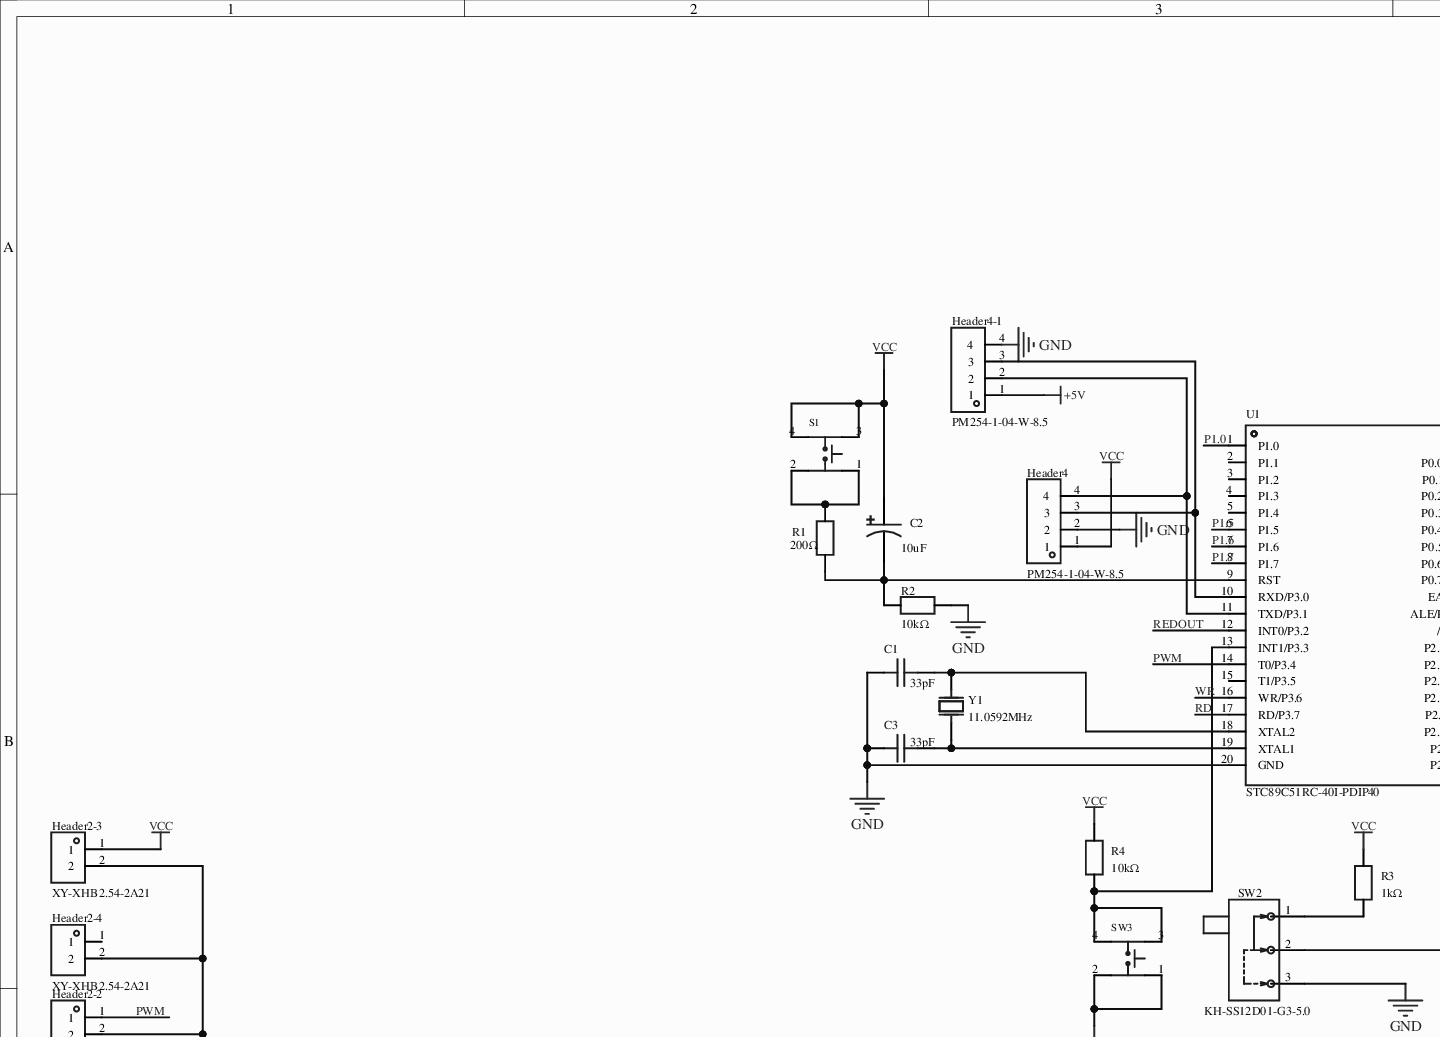
[diagram p0: MISC52142-3.schdoc, top left]
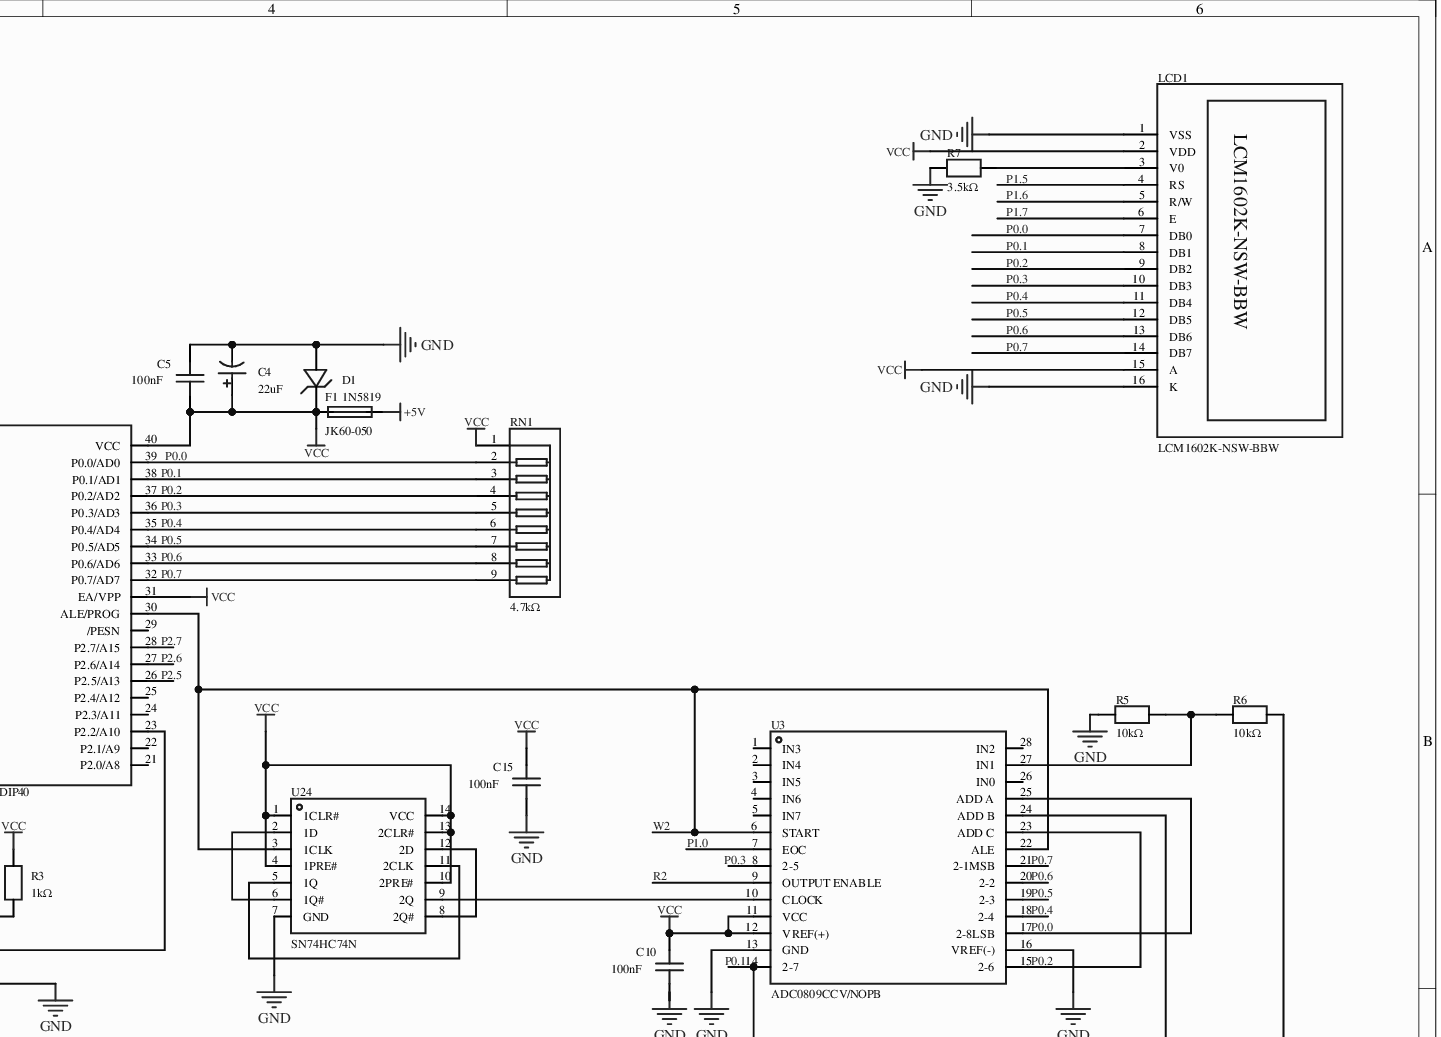
[diagram p1: MISC52142-3.schdoc, top right]
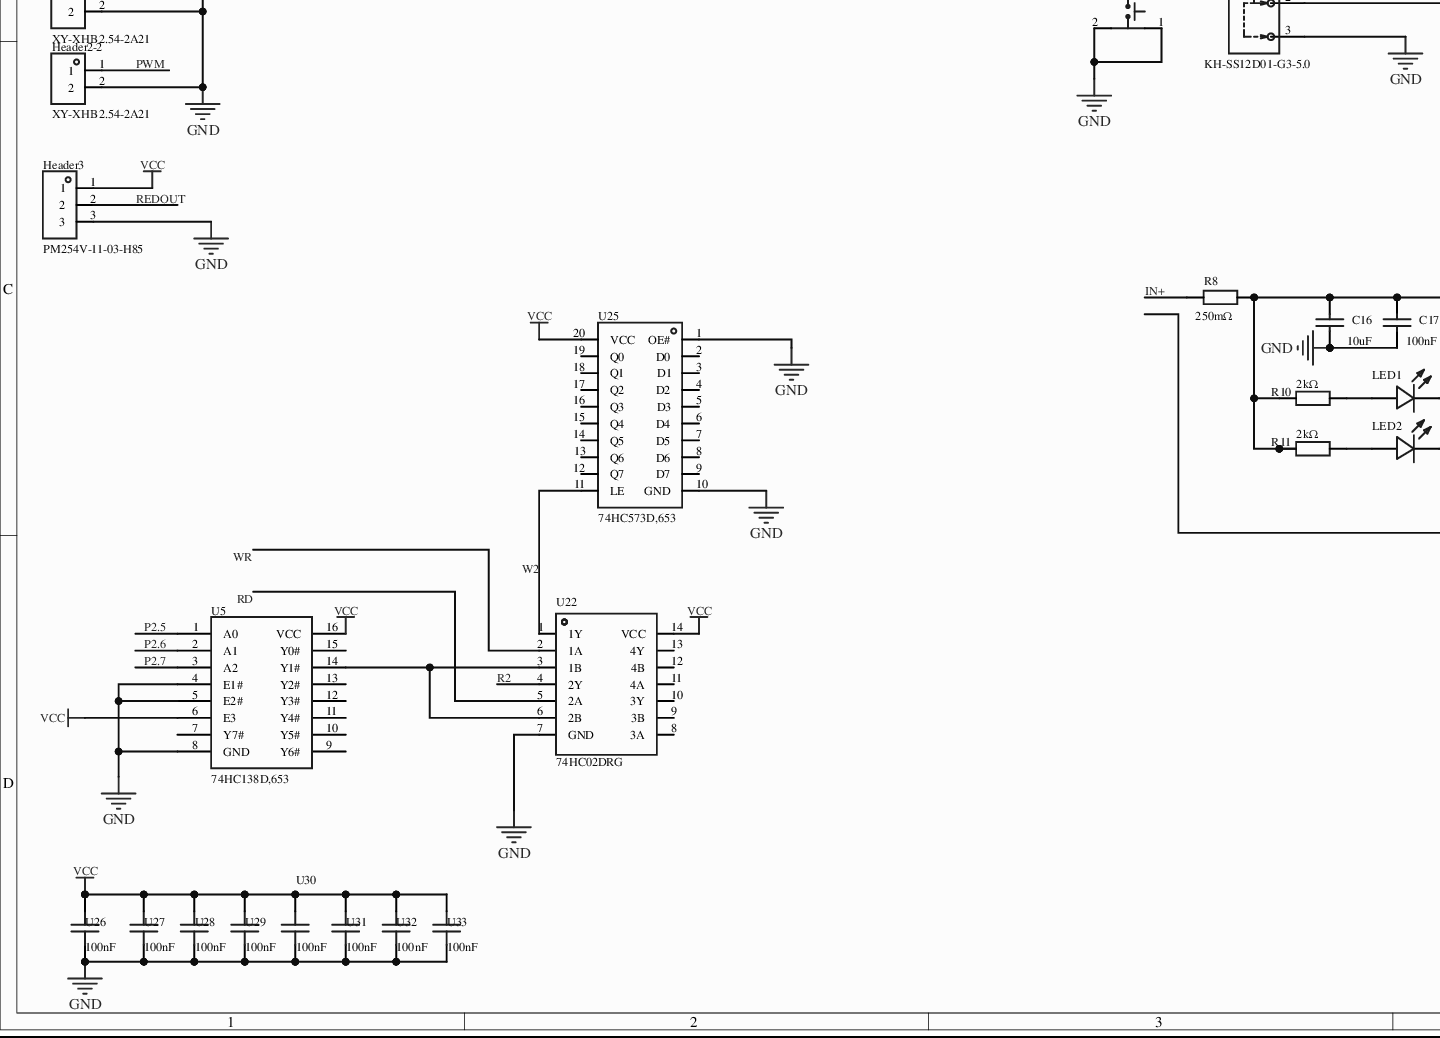
[diagram p2: MISC52142-3.schdoc, bottom left]
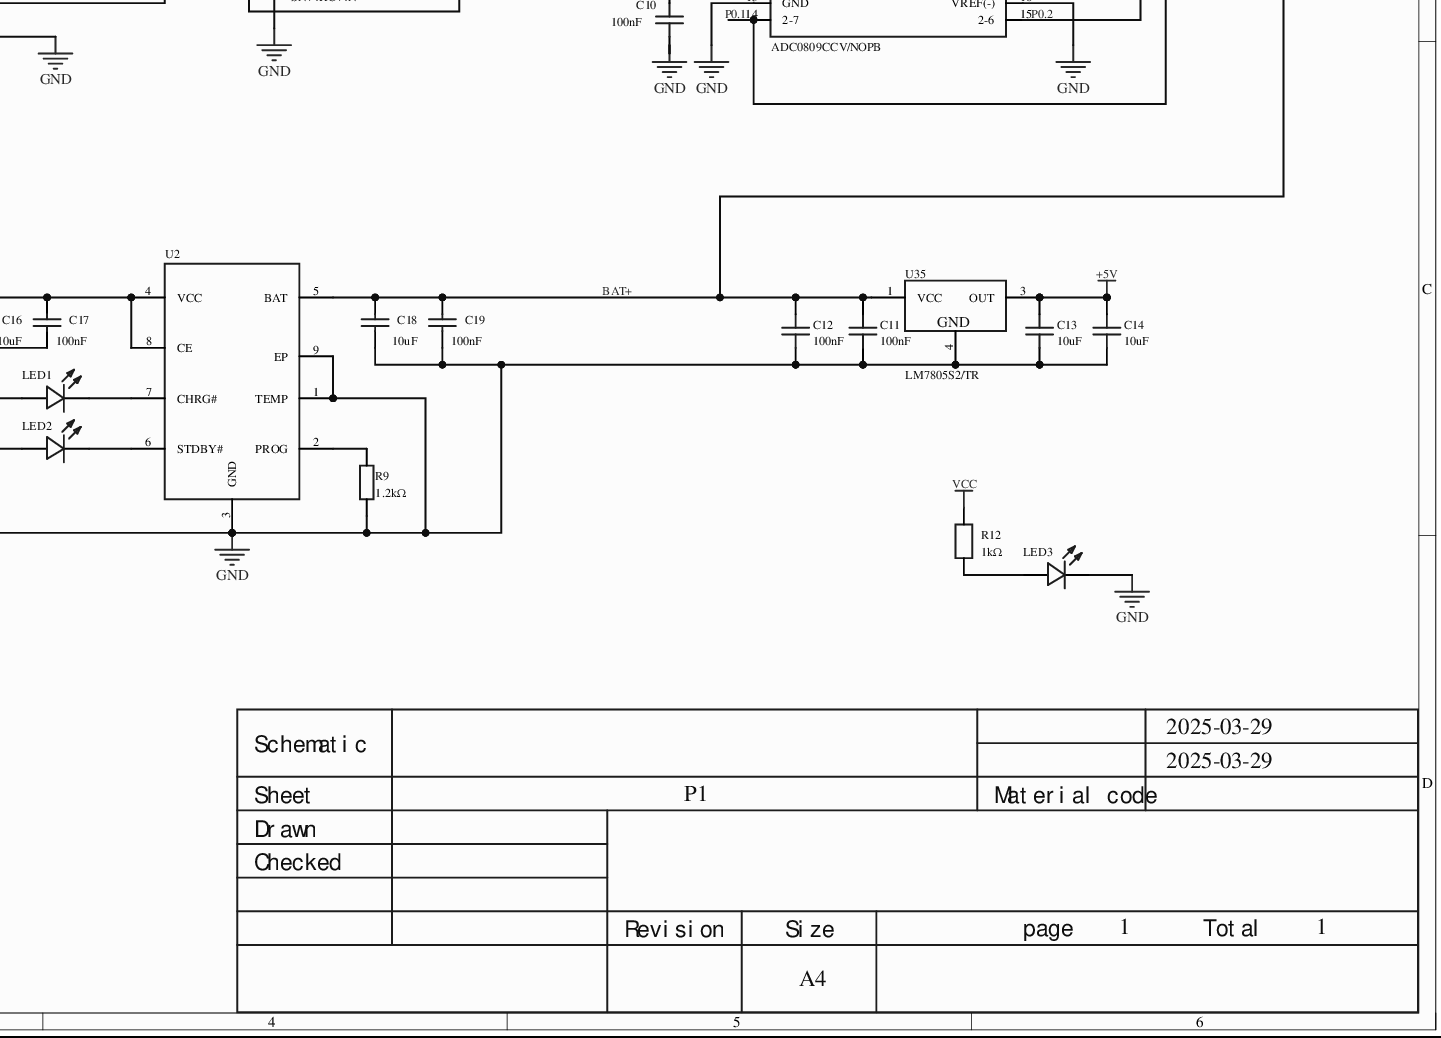
[diagram p3: MISC52142-3.schdoc, bottom right]
# Altium project MISC52142-2.PrjPcb
1 sheet, 60 parts. Net scope: global (net labels, ports and power ports of the same name join across sheets).
Board file: MISC52142.pcbdoc

## Sheet MISC52142-3.schdoc
size 420 x 298 mm; Version: V1.0; @Project Name: MISC52142; @Page Count: 1; @Update Date: 2025-03-29; @Create Date: 2025-03-29; @Schematic Name: MISC52142; @Page No: 1

### Parts
C1  33pF  [RAD-0.2]
C2  10uF  [RB1-2]
C3  33pF  [RAD-0.2]
C4  22uF  [RB1-2]
C5  100nF  [RAD-0.2]
C10  100nF  [RAD-0.2]
C11  100nF  [RAD-0.2]
C12  100nF  [RAD-0.2]
C13  10uF  [RAD-0.2]
C14  10uF  [RAD-0.2]
C15  100nF  [RAD-0.2]
C16  10uF  [RAD-0.2]
C17  100nF  [RAD-0.2]
C18  10uF  [RAD-0.2]
C19  100nF  [RAD-0.2]
D1  1N5819  [DIODE-3]
F1  JK60-050  [FUSE-2]
Header2-2  XY-XHB2.54-2A21  [CON2-5]
Header2-3  XY-XHB2.54-2A21  [CON2-5]
Header2-4  XY-XHB2.54-2A21  [CON2-5]
Header3  PM254V-11-03-H85  [CON3]
Header4  PM254-1-04-W-8.5  [CON4]
Header4-1  PM254-1-04-W-8.5  [CON4]
LCD1  LCM1602K-NSW-BBW  [LCD1602]
LED1  204-10SYGD/S530-E3  [LED1]  (value not drawn)
LED2  333-2SYGD/S530-E2-L  [LED1]  (value not drawn)
LED3  204-10SYGD/S530-E3  [LED1]  (value not drawn)
R1  200Ω  [AXIAL-0.3]
R2  10kΩ  [AXIAL-0.3]
R3  1kΩ  [AXIAL-0.3]
R4  10kΩ  [AXIAL-0.3]
R5  10kΩ  [AXIAL-0.3]
R6  10kΩ  [AXIAL-0.3]
R7  3.5kΩ  [AXIAL-0.3]
R8  250mΩ  [AXIAL-0.3]
R9  1.2kΩ  [AXIAL-0.3]
R10  2kΩ  [AXIAL-0.3]
R11  2kΩ  [AXIAL-0.3]
R12  1kΩ  [AXIAL-0.3]
RN1  4.7kΩ  [RP]
S1  (no value)  [RST]
SW2  KH-SS12D01-G3-5.0  [RT]
SW3  (no value)  [RST]
U1  STC89C51RC-40I-PDIP40  [DIP-40]
U2  TP4056-42-ESOP8  [ESOP-8_L4.9-W3.9-P1.27-LS6.0-BL-EP]  (value not drawn)
U3  ADC0809CCV/NOPB  [DIP-28]
U5  74HC138D,653  [DIP-16]
U22  74HC02DRG  [DIP-14]
U24  SN74HC74N  [DIP-14]
U25  74HC573D,653  [DIP-20]
U26  100nF  [RAD-0.2]
U27  100nF  [RAD-0.2]
U28  100nF  [RAD-0.2]
U29  100nF  [RAD-0.2]
U30  100nF  [RAD-0.2]
U31  100nF  [RAD-0.2]
U32  100nF  [RAD-0.2]
U33  100nF  [RAD-0.2]
U35  LM7805S2/TR  [TO-263-2_L10.0-W9.1-P5.08-LS15.2-BL]
Y1  11.0592MHz  [XTAL-2]

### Nets
+5V: C13.2 C14.2 F1.2 Header4-1.1 U35.3(OUT)
GND: C1.2 C3.2 C4.2 C5.2 C10.1 C11.1 C12.1 C13.1 C14.1 C15.1 C16.1 C17.1 C18.1 C19.1 D1.2(A) Header2-2.2 Header2-3.2 Header2-4.2 Header3.3 Header4.2 Header4-1.4 LCD1.1(VSS) LCD1.16(K) LED3.2(-) R2.2 R5.1 R7.1 R9.1 SW2.3 SW3.1 SW3.2 U1.20(GND) U2.1(TEMP) U2.3(GND) U2.9(EP) U3.13(GND) U3.16(VREF(-)) U5.4(E1#) U5.5(E2#) U5.8(GND) U22.7(GND) U24.7(GND) U25.1(OE#) U25.10(GND) U26.1 U27.1 U28.1 U29.1 U30.1 U31.1 U32.1 U33.1 U35.4(GND)
VCC: C2.1 C4.1 C5.1 C10.2 C15.2 D1.1(C) F1.1 Header2-3.1 Header3.1 Header4.1 LCD1.2(VDD) LCD1.15(A) R3.2 R4.2 R12.2 RN1.1 S1.3 S1.4 U1.31(EA/VPP) U1.40(VCC) U3.11(VCC) U3.12(VREF(+)) U5.6(E3) U5.16(VCC) U22.14(VCC) U24.1(1CLR#) U24.4(1PRE#) U24.10(2PRE#) U24.13(2CLR#) U24.14(VCC) U25.20(VCC) U26.2 U27.2 U28.2 U29.2 U30.2 U31.2 U32.2 U33.2
BAT+: C11.2 C12.2 C18.2 C19.2 R6.2 U2.5(BAT) U35.1(VCC)
IN+: R8.1
P0.0: LCD1.7(DB0) RN1.2 U1.39(P0.0/AD0) U3.17(2-8LSB) U3.25(ADD_A)
P0.1: LCD1.8(DB1) RN1.3 U1.38(P0.1/AD1) U3.14(2-7) U3.24(ADD_B)
P0.2: LCD1.9(DB2) RN1.4 U1.37(P0.2/AD2) U3.15(2-6) U3.23(ADD_C)
P0.3: LCD1.10(DB3) RN1.5 U1.36(P0.3/AD3) U3.8(2-5)
P0.4: LCD1.11(DB4) RN1.6 U1.35(P0.4/AD4) U3.18(2-4)
P0.5: LCD1.12(DB5) RN1.7 U1.34(P0.5/AD5) U3.19(2-3)
P0.6: LCD1.13(DB6) RN1.8 U1.33(P0.6/AD6) U3.20(2-2)
P0.7: LCD1.14(DB7) RN1.9 U1.32(P0.7/AD7) U3.21(2-1MSB)
P1.0: U1.1(P1.0) U3.7(EOC)
P1.5: LCD1.4(RS) U1.6(P1.5)
P1.6: LCD1.5(R/W) U1.7(P1.6)
P1.7: LCD1.6(E) U1.8(P1.7)
P2.5: U1.26(P2.5/A13) U5.1(A0)
P2.6: U1.27(P2.6/A14) U5.2(A1)
P2.7: U1.28(P2.7/A15) U5.3(A2)
PWM: Header2-2.1 U1.14(T0/P3.4)
R2: U3.9(OUTPUT_ENABLE) U22.4(2Y)
RD: U1.17(RD/P3.7) U22.5(2A)
REDOUT: Header3.2 U1.12(INT0/P3.2)
W2: U1.30(ALE/PROG) U3.6(START) U3.22(ALE) U22.1(1Y) U24.3(1CLK) U25.11(LE)
WR: U1.16(WR/P3.6) U22.2(1A)
NetC1_1: C1.1 U1.18(XTAL2) Y1.1(OSC1)
NetC2_2: C2.2 R1.2 R2.1 U1.9(RST)
NetC3_1: C3.1 U1.19(XTAL1) Y1.2(OSC2)
NetC16_2: C16.2 C17.2 R8.2 R10.1 R11.1 U2.4(VCC) U2.8(CE)
NetHeader4_3: Header4.3 Header4-1.3 U1.10(RXD/P3.0)
NetHeader4_4: Header4.4 Header4-1.2 U1.11(TXD/P3.1)
NetLCD1_3: LCD1.3(V0) R7.2
NetLED1_1: LED1.1(+) R10.2
NetLED1_2: LED1.2(-) U2.7(CHRG#)
NetLED2_1: LED2.1(K) U2.6(STDBY#)
NetLED2_2: LED2.2(A) R11.2
NetLED3_1: LED3.1(+) R12.1
NetR1_1: R1.1 S1.1 S1.2
NetR3_1: R3.1 SW2.1
NetR4_1: R4.1 SW3.3 SW3.4 U1.13(INT1/P3.3)
NetR5_2: R5.2 R6.1 U3.27(IN1)
NetR9_2: R9.2 U2.2(PROG)
NetSW2_2: SW2.2 U1.23(P2.2/A10)
NetU3_10: U3.10(CLOCK) U24.9(2Q)
NetU5_14: U5.14(Y1#) U22.3(1B) U22.6(2B)
NetU24_2: U24.2(1D) U24.6(1Q#)
NetU24_5: U24.5(1Q) U24.11(2CLK)
NetU24_8: U24.8(2Q#) U24.12(2D)

Not connected (* = marked no-connect by the designer): Header2-4 1; U1 2(P1.1) 3(P1.2) 4(P1.3) 5(P1.4) 15(T1/P3.5) 21(P2.0/A8) 22(P2.1/A9) 24(P2.3/A11) 25(P2.4/A12) 29(/PESN); U3 1(IN3) 2(IN4) 3(IN5) 4(IN6) 5(IN7) 26(IN0) 28(IN2); U5 7(Y7#) 9(Y6#) 10(Y5#) 11(Y4#) 12(Y3#) 13(Y2#) 15(Y0#); U22 8(3A) 9(3B) 10(3Y) 11(4A) 12(4B) 13(4Y); U25 2(D0) 3(D1) 4(D2) 5(D3) 6(D4) 7(D5) 8(D6) 9(D7) 12(Q7) 13(Q6) 14(Q5) 15(Q4) 16(Q3) 17(Q2) 18(Q1) 19(Q0)

### Notes on the sheet
- 2025-03-29
- Schematic
- Sheet
- P1
- Material code
- Checked
- Drawn
- Revision
- Size
- A4
- page
- 1
- Total

### Library data of the parts
C1 C3 = CC4-0805N330J500F3: Capacitance: 33pF; Tolerance: ±5%; Rated voltage: 50V; Temperature coefficient: C0G;; Manufacturer: FH(风华); AddInBom: yes; ModelId: 5610b656e7164072960d9d2d8c7d4fdf; ModelName: CAP-TH_L4.2-W3.8-H3.8-P5.08; ModelTransform: 222.8342,149.606,0,0,0,0,0,0,-118.11; Symbol: CC4-0805N330J500F3; Device: CC4-0805N330J500F3; Supplier: LCSC; Manufacturer Part: CC4-0805N330J500F3; Value: 33pF; Supplier Part: C94712; JLCPCB Part Class: Extended Part; LCSC Part Name: 33pF ±5% 50V; Supplier Footprint: 插件,P=5.08mm; Datasheet: https://atta.szlcsc.com/upload/public/pdf/source/20190402/C385200_059806A6312B28FF1421A2413EB641E1.pdf; ConvertToPcb: yes; FootprintName: RAD-0.2; Voltage Rated: 50V; Temperature Coefficient: C0G
C2 = KS1C100MB070A00CV0: Capacitance: 10uF; Tolerance: ±20%; Rated voltage: 16V; Ripple current: 24mA@120Hz; ESR: -;; Manufacturer: HUAWEI(华威集团); AddInBom: yes; ModelId: 8017ea3dd4884afab5fc61dd7898abc1; ModelName: CAP-TH_D4.0-H7.0-P1.5; ModelTransform: 158.2674,157.45008,0,0,0,0,0,0,-137.795; φD: 4mm; L: 7mm; Lifetime @ Temp: 1000hrs@105℃; Symbol: KS1C100MB070A00CV0; Device: KS1C100MB070A00CV0; LCSC Part Name: 10uF ±20% 16V; SupplierPart: C216315; ManufacturerPart: KS1C100MB070A00CV0; Supplier Footprint: 插件,D4xL7mm; JLCPCB Part Class: Extended Part; Datasheet: https://atta.szlcsc.com/upload/public/pdf/source/20180905/C271443_A6F66C79EF84E009A061F1FE7B9BC844.pdf; Supplier: LCSC; ConvertToPcb: yes; FootprintName: RB1-2; Value: 10uF; Rated Voltage: 16V; Ripple Current: 24mA@120Hz; Equivalent Series Resistance(ESR): -; Lead Spacing: 1.5mm
C4 = KM226M016D11RR0VH2FP0: Capacitance: 22uF; Tolerance: ±20%; Rated voltage: 16V; Ripple current: -; ESR: -;; Manufacturer: CX(承兴); Symbol: 22uF 16V 5*11; AddInBom: yes; ModelId: edeeed87cbc746108d01291548c38636; ModelName: CAP-TH_D5.0×H7.0×P2.0; ModelTransform: 197.091,196.7911,0,0,0,0,0,0,-137.795; φD: 5mm; L: 11mm; Lifetime @ Temp: 1000hrs@105℃; Device: KM226M016D11RR0VH2FP0; Supplier: LCSC; Manufacturer Part: KM226M016D11RR0VH2FP0; Value: 22uF; Supplier Part: C43844; JLCPCB Part Class: Extended Part; LCSC Part Name: 22uF ±20% 16V; Supplier Footprint: 插件,D5xL11mm; Datasheet: https://atta.szlcsc.com/upload/public/pdf/source/20211027/06D6BA3719C264B639DC286D935D03EA.pdf; ConvertToPcb: yes; FootprintName: RB1-2; Rated Voltage: 16V; Ripple Current: -; Equivalent Series Resistance(ESR): -; Lead Spacing: 2mm
C5 C10 C15 = 178MU0002: Capacitance: 100nF; Tolerance: ±10%; Rated voltage: 50V; Temperature coefficient: X7R;; Manufacturer: KNSCHA(科尼盛); AddInBom: yes; ModelId: 74dcae8ecb8a4760a51624fa9dde4624; ModelName: CAP-TH_L5.8-W3.6-P5.0-D0.6; ModelTransform: 228.346,142.1257,0,0,0,0,0,0,-196.85; Symbol: 178MU0002; Device: 178MU0002; Supplier: LCSC; Supplier Part: C5632426; Manufacturer Part: 178MU0002; Value: 100nF; JLCPCB Part Class: Extended Part; LCSC Part Name: 100nF ±10% 50V; Supplier Footprint: 插件,P=5.08mm; Datasheet: https://atta.szlcsc.com/upload/public/pdf/source/20230506/08E784E6BF236BA57EBA91152AC3AC6D.pdf; ConvertToPcb: yes; FootprintName: RAD-0.2; Voltage Rated: 50V; Temperature Coefficient: X7R
C11 C12 = CC0603KRX7R9BB104: Capacitance: 100nF; Tolerance: ±10%; Rated voltage: 50V; Material (temp. coefficient): X7R;; Manufacturer: YAGEO(国巨); AddInBom: yes; ModelId: ac125912035d415993ca9572d50418b1; ModelName: C0603_L1.6-W0.8-H0.8; ModelTransform: 62.992,31.496,0,0,0,0,0,0,0; Symbol: CC0603KRX7R9BB104; Device: CC0603KRX7R9BB104; Supplier: LCSC; Manufacturer Part: CC0603KRX7R9BB104; Value: 100nF; Supplier Part: C14663; JLCPCB Part Class: Basic Part; LCSC Part Name: 100nF ±10% 50V; Supplier Footprint: 0603; Datasheet: https://atta.szlcsc.com/upload/public/pdf/source/20180910/C282072_33301C7F631E79921B82A8DAC6BCC5B3.pdf; ConvertToPcb: yes; FootprintName: RAD-0.2; Voltage Rated: 50V; Temperature Coefficient: X7R
C13 C14 = CL10A106MQ8NNNC: Capacitance: 10uF; Tolerance: ±20%; Rated voltage: 6.3V; Material (temp. coefficient): X5R;; Manufacturer: SAMSUNG(三星); AddInBom: yes; ModelId: ac125912035d415993ca9572d50418b1; ModelName: C0603_L1.6-W0.8-H0.8; ModelTransform: 62.992,31.496,0,0,0,0,0,0,0; Symbol: CL10A106MQ8NNNC; Device: CL10A106MQ8NNNC; Supplier: LCSC; Manufacturer Part: CL10A106MQ8NNNC; Value: 10uF; Supplier Part: C1691; JLCPCB Part Class: Extended Part; LCSC Part Name: 10uF ±20% 6.3V; Supplier Footprint: 0603; Datasheet: https://atta.szlcsc.com/upload/public/pdf/source/20160218/1457707763339.pdf; ConvertToPcb: yes; FootprintName: RAD-0.2; Voltage Rated: 6.3V; Temperature Coefficient: X5R
C16 C18 = CL21A106KOQNNNE: Capacitance: 10uF; Tolerance: ±10%; Rated voltage: 16V; Material (temp. coefficient): X5R;; Manufacturer: SAMSUNG(三星); Add into BOM: yes; 3D Model: 1ba041120af144c991958decab20d241; 3D Model Transform: 78.74,51.181,0,0,0,0,0,0.0005,0; ModelName: C0805_L2.0-W1.3-H1.3; Symbol: CL21A106KOQNNNE; LCSC Part Name: 10uF ±10% 16V; Supplier Part: C1713; Manufacturer Part: CL21A106KOQNNNE; Supplier Footprint: 0805; JLCPCB Part Class: Extended Part; Datasheet: https://atta.szlcsc.com/upload/public/pdf/source/20160103/1457707694240.pdf; Supplier: LCSC; Convert to PCB: yes; Value: 10uF; Voltage Rated: 16V; Temperature Coefficient: X5R; Device: CL21A106KOQNNNE; FootprintName: RAD-0.2
C17 C19 = CC0805KRX7R9BB104: Capacitance: 100nF; Tolerance: ±10%; Rated voltage: 50V; Material (temp. coefficient): X7R;; Manufacturer: YAGEO(国巨); Add into BOM: yes; 3D Model: 1ba041120af144c991958decab20d241; 3D Model Transform: 78.74,51.181,0,0,0,0,0,0.0005,0; ModelName: C0805_L2.0-W1.3-H1.3; Symbol: CC0805KRX7R9BB104; LCSC Part Name: 100nF ±10% 50V; Supplier Part: C49678; Manufacturer Part: CC0805KRX7R9BB104; Supplier Footprint: 0805; JLCPCB Part Class: Basic Part; Datasheet: https://atta.szlcsc.com/upload/public/pdf/source/20151026/1457707504898.pdf; Supplier: LCSC; Convert to PCB: yes; Value: 100nF; Voltage Rated: 50V; Temperature Coefficient: X7R; Device: CC0805KRX7R9BB104; FootprintName: RAD-0.2
D1 = 1N5819_C402218: Forward voltage drop (Vf): 900mV@3A; DC reverse voltage (Vr): 40V; Average rectified current (Io): 1A;; Manufacturer: LGE(鲁光); AddInBom: yes; ModelId: 6de1e9b71a0d4751b4e9df530304c1a3; ModelName: DO-41_D2.4-L4.7-P8.70; ModelTransform: 374.016,94.488,0,0,0,0,0,0,-137.795; Symbol: 1N5819_C402218; Device: 1N5819_C402218; Supplier: LCSC; Supplier Part: C402218; Manufacturer Part: 1N5819; JLCPCB Part Class: Extended Part; LCSC Part Name: 电压:40V 电流:1A; Supplier Footprint: DO-41; Datasheet: https://atta.szlcsc.com/upload/public/pdf/source/20190705/C402218_ECB4BB85D6DB51BBD80C05504B9336F4.pdf; ConvertToPcb: yes; FootprintName: DIODE-3; Forward Voltage (Vf@If): 900mV@3A; Reverse Voltage (Vr): 40V; Average Rectified Current (Io): 1A
F1 = JK60-050: Max voltage: 60V; Max current: 40A; Hold current: 500mA; Trip current: 1A;; Manufacturer: JK(金科); Symbol: JK60-050_C369084; AddInBom: yes; ModelId: a577626d9dfe4d5a9a614f24ba40a72e; ModelName: FUSE-TH_L7.8-W3.0-P5.1; ModelTransform: 306.809,102.362,0,0,0,0,0,0,-137.795; Power Dissipation: 770mW; Resistance - Initial (Ri) (Min): 400mΩ; Resistance - Post Trip (R1) (Max): 790mΩ; Maximum Time to Trip: 5s; Device: JK60-050; Supplier: LCSC; Supplier Part: C369084; Manufacturer Part: JK60-050; JLCPCB Part Class: Extended Part; LCSC Part Name: 60V 500mA 插件自恢复; Supplier Footprint: 插件,P=5.1mm; Datasheet: https://atta.szlcsc.com/upload/public/pdf/source/20190402/C369097_098D69FB3F8C11406977E7DFA4988746.pdf; ConvertToPcb: yes; FootprintName: FUSE-2; Operating Voltage (Max): 60V; Current Rating (Max): 40A; Hold Current: 500mA; Trip Current: 1A; Operating Temperature: -40℃~+85℃
Header2-2-Header2-4 = XY-XHB2.54-2A21: Pin structure: 1x2P; Pitch: 2.54mm; Mounting: right-angle; Total pins: 2P; Rows: 1; Pins per row: 2; Row spacing: 2.54mm; Rated current: 2A; Operating temperature: -25℃~+85℃;; Manufacturer: XYECONN(辛译); AddInBom: yes; ModelId: 87e1c841624f41b0bf6a09f3d53d2fd2; ModelName: HDR-TH_2P-P2.50-H-F-W7.3-N; ModelTransform: 295.669,304.7238,0,180,0,0,0,-137.795,-133.858; Number of PINs Per Row: 2; Symbol: XY-XHB2.54-2A21; Device: XY-XHB2.54-2A21; LCSC Part Name: 1x2P 间距:2.54mm 弯插; SupplierPart: C19271395; ManufacturerPart: XY-XHB2.54-2A21; Supplier Footprint: 弯插,P=2.54mm; JLCPCB Part Class: Extended Part; Datasheet: https://atta.szlcsc.com/upload/public/pdf/source/20231124/E581531705911B495C6E735B7C4EA3F8.pdf; Supplier: LCSC; ConvertToPcb: yes; FootprintName: CON2-5; Pins Structure: 1x2P; Mounting Style: Right-angle; Number of Pins: 2P; Number of Rows: 1; Row Spacing: 2.54mm; Current Rating (Max): 2A; Operating Temperature Range: -25℃~+85℃
Header3 = PM254V-11-03-H85: Hole structure: 1x3P; Pitch: 2.54mm; Row spacing: -; Mounting: through-hole; Rows: single row; Total holes: 3P; Plastic height: -; Contact material: brass; Contact plating: -;; Manufacturer: XFCN(兴飞); AddInBom: yes; ModelId: f3b3cc5aae9641bf9e56fc160cef875b; ModelName: HDR2.54-F-LI-1X3P; ModelTransform: 299.9994,100,0,0,0,0,0,0,-118.11; Symbol: PM254V-11-03-H85; Device: PM254V-11-03-H85; LCSC Part Name: 间距:2.54mm 1x3P 直插; SupplierPart: C541850; ManufacturerPart: PM254V-11-03-H85; Supplier Footprint: 插件,P=2.54mm; JLCPCB Part Class: Extended Part; Datasheet: https://atta.szlcsc.com/upload/public/pdf/source/20200518/C541849_85853D71FC67C51915A806977A588FDA.pdf; Supplier: LCSC; ConvertToPcb: yes; FootprintName: CON3; Holes Structure: 1x3P; Row Spacing: -; Mounting Type: Through-hole; Number of Rows: Single row; Number of Holes: 3P; Insulation Height: -; Contact Material: Brass; Contact Plating: -
Header4 Header4-1 = PM254-1-04-W-8.5: 插孔结构:1x4P;间距:2.54mm;行距:-;圆孔/方孔:方孔;安装类型:弯插;排数:单排;总孔位数:4P;额定电流:3A;额定电压:-;插孔方向:侧面;塑高:8.5mm;触头材质:铜合金;工作温度范围:-40℃~+105℃;焊接温度(最大值):260℃@5S;; Manufacturer: HCTL(华灿天禄); AddInBom: yes; ModelId: f3aea7e76cee41099dd7459ba1f81f0c; ModelName: HDR-TH_4P-P2.54-H-F-W10.0-N; ModelTransform: 415.7472,419.291,0,0,0,0,0,-196.85,-125.984; Holes Structure: 1x4P; Pitch: 2.54mm; Circular Hole / Square Hole: Square hole; Number of Holes: 4P; Current Rating (Max): 3A; Holes Direction: Side; Symbol: PM254-1-04-W-8.5; Device: PM254-1-04-W-8.5; LCSC Part Name: 1x4P 间距:2.54mm 弯插; SupplierPart: C2897386; ManufacturerPart: PM254-1-04-W-8.5; Supplier Footprint: 弯插,P=2.54mm; JLCPCB Part Class: Extended Part; Datasheet: https://atta.szlcsc.com/upload/public/pdf/source/20230609/7BA40A3D721268A082DCDEAD4C99131B.pdf; Supplier: LCSC; ConvertToPcb: yes; FootprintName: CON4; Row Spacing: -; Mounting Type: Right-angle; Number of Rows: Single row; Voltage Rating (Max): -; Insulation Height: 8.5mm; Contact Material: Copper alloy; Operating Temperature Range: -40℃~+105℃; Soldering Temperature(Max): 260℃@5S
LCD1 = LCM1602K-NSW-BBW: Main controller chip: KS0066U; Size (inch): -;; Manufacturer: LONTECH(厦门龙特); AddInBom: yes; ModelId: 84dc4c036e12490da40aa0593fb5d02d; ModelName: MODULE-TH_LCM1602K; ModelTransform: 3149.6,1417.32,0,0,0,0,509.803,-610.157,0; Symbol: LCM1602K-NSW-BBW; Device: LCM1602K-NSW-BBW; LCSC Part Name: LCM1602K-NSW-BBW; SupplierPart: C83275; ManufacturerPart: LCM1602K-NSW-BBW; Supplier Footprint: -; JLCPCB Part Class: Extended Part; Datasheet: https://atta.szlcsc.com/upload/public/pdf/source/20161111/1478835376580.pdf; Supplier: LCSC; ConvertToPcb: yes; FootprintName: LCD1602; Main Control Chip: KS0066U; Size: -
LED1 = 204-10SYGD/S530-E3: Lamp head type: 3mm round lamp head; Emitted color: yellow-green;; Manufacturer: EVERLIGHT(亿光); Symbol: SZYY0805R; Add into BOM: yes; 3D Model: 7a5158147ccf41a18926a05cf5a7749d; 3D Model Transform: 139.516,157.15173,0,0,0,0,-9.054,-1.181,-137.795; Lens Color: Water clear; Dominant Wavelength: 615nm~630nm; Peak Wavelength: 645nm; Forward Current: 10mA; Power Dissipation: 40mW; Viewing Angle: 120°; PinNumber: LED1(1,2); ModelName: LED-TH_BD3.8-P2.54-FD; LCSC Part Name: 普绿/黄绿; Supplier Part: C85161; Manufacturer Part: 204-10SYGD/S530-E3; Supplier Footprint: 插件,D=3mm; JLCPCB Part Class: Extended Part; Datasheet: https://atta.szlcsc.com/upload/public/pdf/source/20181205/C85161_54D2881904BBFDED7AAB4D08F0D96F46.pdf; Supplier: LCSC; Convert to PCB: yes; Emitted Color: Yellow-green; Diode Configuration: -; Color Temperature: -; Mounting Sytle: -; Operating Temperature: -40℃~+85℃; Device: 204-10SYGD/S530-E3; FootprintName: LED1; Lamp Holder Type: 3mm round lamp head
LED2 = 333-2SYGD/S530-E2-L: 灯头类型:5mm圆形灯头;发光颜色:黄绿色;功率:60mW;正向电流:20mA;主波长:573nm;二极管配置:-;透镜颜色:雾状绿透镜;色温:-;发光角度:45°;载带方式:-;工作温度:-40℃~+85℃;; Manufacturer: EVERLIGHT(亿光); Symbol: 17-21SYGC/S530-E3/TR8; Add into BOM: yes; 3D Model: b322f11ad7274358b77d0ea2f14da52e; 3D Model Transform: 214.9602,232.069,0,0,0,0,-8.858,0,-196.85; Emitted Color: Yellow-green; PinNumber: LED2(1,2); ModelName: LED-TH_BD5.0-P2.54-FD; Lamp Holder Type: 5mm round lamp head; Power Dissipation: 60mW; Forward Current: 20mA; Dominant Wavelength: 573nm; Peak Wavelength: 575nm; Lens Color: Diffused green lens; Viewing Angle: 45°; LCSC Part Name: 普绿/黄绿; Supplier Part: C99697; Manufacturer Part: 333-2SYGD/S530-E2-L; Supplier Footprint: 插件,D=5mm; JLCPCB Part Class: Extended Part; Datasheet: https://atta.szlcsc.com/upload/public/pdf/source/20170428/1493376834720.pdf; Supplier: LCSC; Convert to PCB: yes; Device: 333-2SYGD/S530-E2-L; FootprintName: LED1; Diode Configuration: -; Color Temperature: -; Mounting Sytle: -; Operating Temperature: -40℃~+85℃
LED3 = 204-10SYGD/S530-E3: Lamp head type: 3mm round lamp head; Emitted color: yellow-green;; Manufacturer: EVERLIGHT(亿光); Symbol: SZYY0805R; Add into BOM: yes; 3D Model: 7a5158147ccf41a18926a05cf5a7749d; 3D Model Transform: 139.516,157.15173,0,0,0,0,-9.054,-1.181,-137.795; Lens Color: Water clear; Dominant Wavelength: 615nm~630nm; Peak Wavelength: 645nm; Forward Current: 10mA; Power Dissipation: 40mW; Viewing Angle: 120°; PinNumber: LED3(1,2); ModelName: LED-TH_BD3.8-P2.54-FD; LCSC Part Name: 普绿/黄绿; Supplier Part: C85161; Manufacturer Part: 204-10SYGD/S530-E3; Supplier Footprint: 插件,D=3mm; JLCPCB Part Class: Extended Part; Datasheet: https://atta.szlcsc.com/upload/public/pdf/source/20181205/C85161_54D2881904BBFDED7AAB4D08F0D96F46.pdf; Supplier: LCSC; Convert to PCB: yes; Emitted Color: Yellow-green; Diode Configuration: -; Color Temperature: -; Mounting Sytle: -; Operating Temperature: -40℃~+85℃; Device: 204-10SYGD/S530-E3; FootprintName: LED1; Lamp Holder Type: 3mm round lamp head
R1 = MF2WS-200Ω±1%T: Resistor type: Metal film resistor; Resistance: 200Ω; Tolerance: ±1%; Power: 2W; Temperature coefficient: ±200ppm/℃;; Manufacturer: 华星机电; AddInBom: yes; ModelId: 9feba23d1d1b47a8a9d207b2912318fc; ModelName: RES-TH_BD5.0-L15.5-P19.50-D0.8; ModelTransform: 799.21108,196.3,0,0,0,0,0,0,-196.85; Symbol: MF2WS-200Ω±1%T; Device: MF2WS-200Ω±1%T; LCSC Part Name: 金属膜电阻 200Ω ±1% 2W; SupplierPart: C714576; ManufacturerPart: MF2WS-200Ω±1%T; Supplier Footprint: 插件; JLCPCB Part Class: Extended Part; Datasheet: https://atta.szlcsc.com/upload/public/pdf/source/20200731/C713882_AE8EB1102749D7E4FB4FB13DC898C429.pdf; Supplier: LCSC; ConvertToPcb: yes; FootprintName: AXIAL-0.3; Type: Metal film resistor; Value: 200Ω; Power(Watts): 2W; Temperature Coefficient: ±200ppm/℃
R2 R4-R6 = RN1/4W10KFT/BA1: Resistor type: Metal film resistor; Resistance: 10kΩ; Tolerance: ±1%; Power: 250mW; Temperature coefficient: ±50ppm/℃;; Manufacturer: Tyohm(幸亚电阻); AddInBom: yes; ModelId: 463263665006444ab7a47bd11b0cf956; ModelName: RES-TH_BD2.4-L6.3-P10.30-D0.6; ModelTransform: 427.165,94.32816,0,0,0,0,0,0,-196.85; Overload Voltage (Max): 250V; Symbol: RN 1/4W 10K F T/B A1; Device: RN1/4W10KFT/BA1; LCSC Part Name: 10kΩ ±1% 250mW 金属膜电阻; SupplierPart: C410695; ManufacturerPart: RN1/4W10KFT/BA1; Supplier Footprint: 插件; JLCPCB Part Class: Extended Part; Datasheet: https://atta.szlcsc.com/upload/public/pdf/source/20190808/C410699_D126E64D28B638F1D73B58E9F61DFD9B.pdf; Supplier: LCSC; ConvertToPcb: yes; FootprintName: AXIAL-0.3; Type: Metal film resistor; Value: 10kΩ; Power(Watts): 250mW; Temperature Coefficient: ±50ppm/℃; Operating Temperature Range: -55℃~+125℃
R3 R12 = MF1/4W-1KΩ±1%T52: Resistor type: Metal film resistor; Resistance: 1kΩ; Tolerance: ±1%; Power: 250mW; Temperature coefficient: ±200ppm/℃;; Manufacturer: 华星机电; AddInBom: yes; ModelId: 8e6c7ee8323443d1ab8f0504b6353c8c; ModelName: RES-TH_D2.3-L6.5-P10.50; ModelTransform: 431.1015,91.3384,0,0,0,0,0.197,0,-137.795; Symbol: MF1/4W-1KΩ±1%T52; Device: MF1/4W-1KΩ±1%T52; LCSC Part Name: 金属膜电阻 1kΩ ±1% 250mW; SupplierPart: C713997; ManufacturerPart: MF1/4W-1KΩ±1%T52; Supplier Footprint: 插件; JLCPCB Part Class: Extended Part; Datasheet: https://atta.szlcsc.com/upload/public/pdf/source/20200731/C713882_AE8EB1102749D7E4FB4FB13DC898C429.pdf; Supplier: LCSC; ConvertToPcb: yes; FootprintName: AXIAL-0.3; Type: Metal film resistor; Value: 1kΩ; Power(Watts): 250mW; Temperature Coefficient: ±200ppm/℃
R7 = MF1/8W-3K5±1%-ST52: Resistor type: Metal film resistor; Resistance: 3.5kΩ; Tolerance: ±1%; Power: 125mW; Temperature coefficient: ±100ppm/℃;; Manufacturer: VO(翔胜); AddInBom: yes; ModelId: 5631a15c8fe642639fec94924741e635; ModelName: RES-TH_BD2.3-L3.7-P7.62-D0.4; ModelTransform: 316.9285,90.48368,0,0,0,0,0,0,-137.795; Overload Voltage (Max): 200V; Symbol: MF1/8W-3K5±1%-ST52; Device: MF1/8W-3K5±1%-ST52; LCSC Part Name: 金属膜电阻 3.5kΩ ±1% 125mW; SupplierPart: C2903355; ManufacturerPart: MF1/8W-3K5±1%-ST52; Supplier Footprint: 插件,D2.3xL3.7mm; JLCPCB Part Class: Extended Part; Datasheet: https://atta.szlcsc.com/upload/public/pdf/source/20200609/C601728_5AA4C0C8E12E11069DA2C3356F29D1F2.pdf; Supplier: LCSC; ConvertToPcb: yes; FootprintName: AXIAL-0.3; Type: Metal film resistor; Value: 3.5kΩ; Power(Watts): 125mW; Temperature Coefficient: ±100ppm/℃; Operating Temperature Range: -55℃~+155℃
R8 = 25121WF250LT4E: Resistor type: Thick film resistor; Resistance: 250mΩ; Tolerance: ±1%; Power: 1W; Temperature coefficient: ±800ppm/℃; Max working voltage: 200V; Operating temperature: -55℃~+155℃;; Manufacturer: UNI-ROYAL(厚声); AddInBom: yes; ModelId: 954b67263d9e4f3582d8de3f8c846421; ModelName: R2512_L6.3-W3.2-H0.6; ModelTransform: 248.031,125.984,0,0,0,0,-0.0005,0,0; Symbol: 25121WF250LT4E; Device: 25121WF250LT4E; LCSC Part Name: 250mΩ ±1% 1W; SupplierPart: C25467; ManufacturerPart: 25121WF250LT4E; Supplier Footprint: 2512; JLCPCB Part Class: Extended Part; Datasheet: https://atta.szlcsc.com/upload/public/pdf/source/20200306/C422600_1E6D84923E4A46A82E41ADD87F860B5C.pdf; Supplier: LCSC; ConvertToPcb: yes; FootprintName: AXIAL-0.3; Type: Thick film resistor; Value: 250mΩ; Power(Watts): 1W; Temperature Coefficient: ±800ppm/℃; Overload Voltage (Max): 200V; Operating Temperature Range: -55℃~+155℃
R9 = 0805W8F1201T5E: Resistor type: Thick film resistor; Resistance: 1.2kΩ; Tolerance: ±1%; Power: 125mW; Temperature coefficient: ±100ppm/℃; Max working voltage: 150V; Operating temperature: -55℃~+155℃;; Manufacturer: UNI-ROYAL(厚声); Add into BOM: yes; 3D Model: 37a81e68749a4138bd2dfa6897b24b85; 3D Model Transform: 78.74,51.181,0,0,0,0,0,-0.0005,0; ModelName: R0805_L2.0-W1.3-H0.6; Symbol: 0805W8F1201T5E; LCSC Part Name: 1.2kΩ ±1% 125mW; Supplier Part: C17379; Manufacturer Part: 0805W8F1201T5E; Supplier Footprint: 0805; JLCPCB Part Class: Basic Part; Datasheet: https://atta.szlcsc.com/upload/public/pdf/source/20200306/C422600_1E6D84923E4A46A82E41ADD87F860B5C.pdf; Supplier: LCSC; Convert to PCB: yes; Type: Thick film resistor; Value: 1.2kΩ; Power(Watts): 125mW; Temperature Coefficient: ±100ppm/℃; Overload Voltage (Max): 150V; Operating Temperature Range: -55℃~+155℃; Device: 0805W8F1201T5E; FootprintName: AXIAL-0.3
R10 R11 = 0805W8F2001T5E: Resistor type: Thick film resistor; Resistance: 2kΩ; Tolerance: ±1%; Power: 125mW; Temperature coefficient: ±100ppm/℃; Max working voltage: 150V; Operating temperature: -55℃~+155℃;; Manufacturer: UNI-ROYAL(厚声); AddInBom: yes; ModelId: 37a81e68749a4138bd2dfa6897b24b85; ModelName: R0805_L2.0-W1.3-H0.6; ModelTransform: 78.74,51.181,0,0,0,0,0,-0.0005,0; Symbol: 0805W8F2001T5E; Device: 0805W8F2001T5E; LCSC Part Name: 2kΩ ±1% 125mW; SupplierPart: C17604; ManufacturerPart: 0805W8F2001T5E; Supplier Footprint: 0805; JLCPCB Part Class: Basic Part; Datasheet: https://atta.szlcsc.com/upload/public/pdf/source/20200306/C422600_1E6D84923E4A46A82E41ADD87F860B5C.pdf; Supplier: LCSC; ConvertToPcb: yes; FootprintName: AXIAL-0.3; Type: Thick film resistor; Value: 2kΩ; Power(Watts): 125mW; Temperature Coefficient: ±100ppm/℃; Overload Voltage (Max): 150V; Operating Temperature Range: -55℃~+155℃
RN1 = A09-472JP: Resistor count: 8; Resistance: 4.7kΩ; Tolerance: ±5%; Power per element: 125mW; Temperature coefficient: ±100ppm/℃;; Manufacturer: FH(风华); AddInBom: yes; ModelId: d106c67f29e14d8080ba548247a719a1; ModelName: SIP-9_L22.8-W3.0-H8.5-P2.54; ModelTransform: 917.49722,118.11,0,0,0,0,0,0,-137.795; Number of Resistors: 8; Symbol: A09-472JP; Device: A09-472JP; LCSC Part Name: 4.7kΩ ±5%; SupplierPart: C9112; ManufacturerPart: A09-472JP; Supplier Footprint: SIP-9-2.54mm; JLCPCB Part Class: Extended Part; Datasheet: https://atta.szlcsc.com/upload/public/pdf/source/20181127/C336620_2E84FA9E7B5BF76546BC661699514FB8.pdf; Supplier: LCSC; ConvertToPcb: yes; FootprintName: RP; Value: 4.7kΩ; Power(Watts): 125mW; Temperature Coefficient: ±100ppm/℃; Number of Pins: 9
S1 SW3 = SKHHAKA010: Circuit: SPST; Button shape: round button; Mounting: through-hole; Switch length: 6mm; Switch width: 6mm; Switch height: 5mm; Contact current: 50mA; Rated voltage (DC): 12V; Illuminated: -; Mechanical life: -;; Manufacturer: ALPSALPINE(阿尔卑斯阿尔派); AddInBom: yes; ModelId: 20eee248bc684ccd8cbdbb1d0d91ec6f; ModelName: SW-TH_4P-L6.0-W6.0-H5.0-LS6.5-P4.50; ModelTransform: 236.22,323.03,0,90,0,0,0,0,-137.795; Symbol: SKHHAKA010; Device: SKHHAKA010; Supplier: LCSC; Supplier Part: C139754; JLCPCB Part Class: Extended Part; LCSC Part Name: 6*6*5mm 直插 轻触开关; Supplier Footprint: 插件; Datasheet: https://atta.szlcsc.com/upload/public/pdf/source/20180118/C139754_15162575378021279461.pdf; ConvertToPcb: yes; FootprintName: RST; Actuator Style: Round button; Mounting Style: Through-hole; Switch Length: 6mm; Switch Width: 6mm; Switch Height: 5mm; Contact Current: 50mA; Voltage Rating (DC): 12V; With Lamp: -; Mechanical Life: -
SW2 = KH-SS12D01-G3-5.0: Manufacturer: kinghelm(金航标); AddInBom: yes; ModelId: 26d5331bbd27478083cc9b7d4df92690; ModelName: SW-TH_KH-SS12D01-G3-5.0; ModelTransform: 342.519,146.0627,0,0,0,0,-0.005,0,-177.165; Symbol: KH-SS12D01-G3-5.0; Device: KH-SS12D01-G3-5.0; Supplier: LCSC; Supplier Part: C5274456; Manufacturer Part: KH-SS12D01-G3-5.0; JLCPCB Part Class: Extended Part; LCSC Part Name: 拨动开关 KH-SS12D01-G3-5.0针(SS12D00); Supplier Footprint: 插件; Datasheet: https://atta.szlcsc.com/upload/public/pdf/source/20221118/89F8282F9CF9F25DF0FDDB8FDD97EC5C.pdf; ConvertToPcb: yes; FootprintName: RT
U1 = STC89C51RC-40I-PDIP40: Manufacturer: STC(宏晶); AddInBom: yes; ModelId: 16d4686a009b4ddca948f91eddb57b14; ModelName: DIP-40_L52.3-W13.8-H4.0-LS15.24-P2.54; ModelTransform: 2059.051,615.743,0,0,0,0,0,0,-129.921; Symbol: STC89C51RC-40I-PDI; Device: STC89C51RC-40I-PDIP40; Supplier: LCSC; Manufacturer Part: STC89C51RC-40I-PDIP40; Supplier Part: C29286; JLCPCB Part Class: Extended Part; LCSC Part Name: STC89C51RC-40I-PDIP40 停产; Supplier Footprint: DIP-40; Datasheet: https://atta.szlcsc.com/upload/public/pdf/source/20210111/C29286_8D18B35F9C74B93E8391CB56D361E797.pdf; ConvertToPcb: yes; FootprintName: DIP-40
U2 = TP4056-42-ESOP8: Battery type: -; Battery cells: -; Max charge current: -; Full-charge voltage: -; Max supply voltage: -;; Manufacturer: TOPPOWER(南京拓微); Symbol: TP4056; AddInBom: yes; ModelId: d3e00daa36c445139c055a3b9efb85d2; ModelName: ESOP-8_L4.9-W3.9-H1.6-LS6.0-P1.27; ModelTransform: 240.157,192.913,0,90,0,0,0,0,0; Device: TP4056-42-ESOP8; LCSC Part Name: TP4056-42-ESOP8; SupplierPart: C16581; ManufacturerPart: TP4056-42-ESOP8; Supplier Footprint: ESOP-8; JLCPCB Part Class: Basic Part; Datasheet: https://atta.szlcsc.com/upload/public/pdf/source/20190626/C16581_611BCF5D7CF554EAE465137A8F68DB3E.pdf; Supplier: LCSC; ConvertToPcb: yes; FootprintName: ESOP-8_L4.9-W3.9-P1.27-LS6.0-BL-EP; Battery Chemistry: -; Number of Cells: -; Charge Current - Max: -; Battery Pack Voltage: -; Voltage - Supply (Max): -; Interface: -
U3 = ADC0809CCV/NOPB: Interface: parallel; Supply voltage: 4.5V~6.5V; Sampling rate: 10kHz; Resolution: 8-bit;; Manufacturer: TI(德州仪器); AddInBom: yes; ModelId: 0530a8ac3b1240f49986b10b32810c9d; ModelName: PLCC-28_L11.5-W11.5-P1.27-LS12.5-L; ModelTransform: 489.763,489.763,0,0,0,0,0,0,0; number of channels: 8; Symbol: ADC0809CCV/NOPB; Device: ADC0809CCV/NOPB; Supplier: LCSC; Supplier Part: C701070; Manufacturer Part: ADC0809CCV/NOPB; JLCPCB Part Class: Extended Part; LCSC Part Name: ADC0809CCV/NOPB; Supplier Footprint: PLCC-28(11.5x11.5); ConvertToPcb: yes; FootprintName: DIP-28; Interface: Parallel; Supply Voltage: 4.5V~6.5V; sampling frequency: 10kHz; resolution: 8-bit; Operating Temperature: -40℃~+85℃
U5 = 74HC138D,653: Supply voltage: 2V~6V; Channels: 3~8; Sink current (IOL): 5.2mA; Source current (IOH): 5.2mA;; Manufacturer: Nexperia(安世); AddInBom: yes; ModelId: c21ec766ec2643efb3352f8441994f4e; ModelName: SOIC-16_L9.9-W3.9-H1.8-LS6.0-P1.27; ModelTransform: 389.763,236.454,0,0,0,0,0,0,0; Voltage Supply Source: Single supply; Symbol: 74HC138D,653; Device: 74HC138D,653; LCSC Part Name: 74HC138D,653; SupplierPart: C5602; ManufacturerPart: 74HC138D,653; Supplier Footprint: SOIC-16; JLCPCB Part Class: Extended Part; Datasheet: https://atta.szlcsc.com/upload/public/pdf/source/20160918/1474193369767.pdf; Supplier: LCSC; ConvertToPcb: yes; FootprintName: DIP-16; Type: Decoder/Demultiplexer; Supply Voltage: 2V~6V; Number of lines: 3~8; Sink Current: 5.2mA; Source Current: 5.2mA; Operating temperature: -40℃~+125℃
U22 = 74HC02DRG: Logic type: NOR gate; Channels: 4;; Manufacturer: HGC(深圳汉芯); AddInBom: yes; ModelId: 520b569c4a2341089bdfdd9bf52b8619; ModelName: SOP-14_L8.6-W3.9-P1.27-LS6.0-BL; ModelTransform: 339.763,236.22,0,0,0,0,0,0,0; Number of Channels: 4; Symbol: 74HC02DRG; Device: 74HC02DRG; LCSC Part Name: 74HC02DRG; SupplierPart: C5145448; ManufacturerPart: 74HC02DRG; Supplier Footprint: SOP-14L; JLCPCB Part Class: Extended Part; Datasheet: https://atta.szlcsc.com/upload/public/pdf/source/20221024/6DBCB603169C2E0D36701B5C85B467CE.pdf; Supplier: LCSC; ConvertToPcb: yes; FootprintName: DIP-14; Logic Gate Type: NOR gate; Series: 74HC series
U24 = SN74HC74N: Type: D-type; Supply voltage: 2V~6V; Clock frequency: 60MHz; Elements: 2; Bits per element: 1; Max propagation delay: 30ns@6V,50pF; Quiescent current (Iq): 4uA;; Manufacturer: TI(德州仪器); AddInBom: yes; ModelId: ca4ed987146b49a5a2d3ca847d6466c4; ModelName: PDIP-14_L19.3-W6.4-P2.54-LS7.6-BL; ModelTransform: 755.904,309.842,0,0,0,0,0,0,-125.984; Trigger Type: Rising edge; Function: Set and reset; Number of Elements: 2; Number of Bits per Element: 1; Output Type: Complementary; Sink Current: 5.2mA; Input Capacitance: 3pF; Symbol: SN74HC74N; Device: SN74HC74N; LCSC Part Name: SN74HC74N; SupplierPart: C2895; ManufacturerPart: SN74HC74N; Supplier Footprint: DIP-14; JLCPCB Part Class: Extended Part; Supplier: LCSC; ConvertToPcb: yes; FootprintName: DIP-14; Supply Voltage: 2V~6V; Clock Frequency: 60MHz; Maximum Propagation Delay: 30ns@6V,50pF; Series: 74HC series; Source Current: 5.2mA; Quiescent Current (Iq): 4uA; Operating Temperature: -40℃~+85℃
U25 = 74HC573D,653: Logic type: D-type latch; Supply voltage: 2V~6V; Propagation delay: 14ns;; Manufacturer: Nexperia(安世); AddInBom: yes; ModelId: e53fe72ca93a4d7bade5640f2542b411; ModelName: SO-20_L12.8-W7.5-H2.5-P1.27-LS10.3-BL; ModelTransform: 503.936,405.511,0,0,0,0,0,0,0; Output Type: Tri-state; Source Current: 7.8mA; Symbol: 74HC573D,653; Device: 74HC573D,653; LCSC Part Name: 三态输出八路D型锁存器; SupplierPart: C5608; ManufacturerPart: 74HC573D,653; Supplier Footprint: SOIC-20-300mil; JLCPCB Part Class: Extended Part; Datasheet: https://atta.szlcsc.com/upload/public/pdf/source/20190910/C426702_CB3AB1BF1FFE83D27D68962795A0A43F.pdf; Supplier: LCSC; ConvertToPcb: yes; FootprintName: DIP-20; Logic Type: D-type latch; Supply Voltage: 2V~6V; Sink Current: 7.8mA; Propagation Delay: 14ns; OperatingTemperature: -40℃~+125℃
U26-U33 = 178MU0006: Capacitance: 100nF; Tolerance: ±10%; Rated voltage: 50V; Temperature coefficient: X7R;; Manufacturer: KNSCHA(科尼盛); AddInBom: yes; ModelId: 4b9f6362efb04e9bb8d1049df17027a2; ModelName: CAP-TH_L4.2-W3.5-P2.54-D0.5; ModelTransform: 165.354,137.788,0,0,0,0,0,0,-196.85; Symbol: 178MU0006; Device: 178MU0006; LCSC Part Name: 100nF ±10% 50V; SupplierPart: C5632430; ManufacturerPart: 178MU0006; Supplier Footprint: 插件,P=2.54mm; JLCPCB Part Class: Extended Part; Datasheet: https://atta.szlcsc.com/upload/public/pdf/source/20230506/6B3136079A6D587E863927628E877AC6.pdf; Supplier: LCSC; ConvertToPcb: yes; FootprintName: RAD-0.2; Value: 100nF; Voltage Rated: 50V; Temperature Coefficient: X7R
U35 = LM7805S2/TR: Manufacturer: HGSEMI(华冠); AddInBom: yes; ModelId: 0ac16cc0e1a446efb6544455ccf5dafd; ModelName: TO-263-2_L10.0-W9.1-H4.4-LS14.0-P5.08; ModelTransform: 393.7,533.922,0,0,0,0,0,59.056,0; Symbol: LM7805S2/TR; Device: LM7805S2/TR; LCSC Part Name: LM7805S2/TR; SupplierPart: C2902505; ManufacturerPart: LM7805S2/TR; Supplier Footprint: TO-263-2; JLCPCB Part Class: Extended Part; Datasheet: https://atta.szlcsc.com/upload/public/pdf/source/20211025/81B2DEEFFF7C2ADEC3E836E1284744FB.pdf; Supplier: LCSC; ConvertToPcb: yes; FootprintName: TO-263-2_L10.0-W9.1-P5.08-LS15.2-BL
Y1 = X49SD110592MSD2SC: Crystal type: through-hole crystal; Frequency: 11.0592MHz; Frequency tolerance (room temp): ±20ppm; Load capacitance: 20pF; Frequency stability (full temp): ±30ppm;; Manufacturer: YXC(扬兴晶振); AddInBom: yes; ModelId: a8e34f6c394c4d60ace7720f62d1ccdf; ModelName: HC-49US_L11.0-W4.5-H3.5-P4.88; ModelTransform: 432.46488,177.165,0,0,0,0,0,0,-137.795; Symbol: X49SD110592MSD2SC; Device: X49SD110592MSD2SC; LCSC Part Name: 11.0592MHz ±20ppm 20pF; SupplierPart: C2203; ManufacturerPart: X49SD110592MSD2SC; Supplier Footprint: HC-49S; JLCPCB Part Class: Extended Part; Datasheet: https://atta.szlcsc.com/upload/public/pdf/source/20240329/977D7F2434F98B2BE33270BB9FF3D86D.pdf; Supplier: LCSC; ConvertToPcb: yes; FootprintName: XTAL-2; Crystal Type: Through-hole crystal; Value: 11.0592MHz; Normal temperature Frequency Tolerance: ±20ppm; External load capacitor: 20pF; Frequency Stability(Full temperature range): ±30ppm; Operating Temperature: -20℃~+70℃